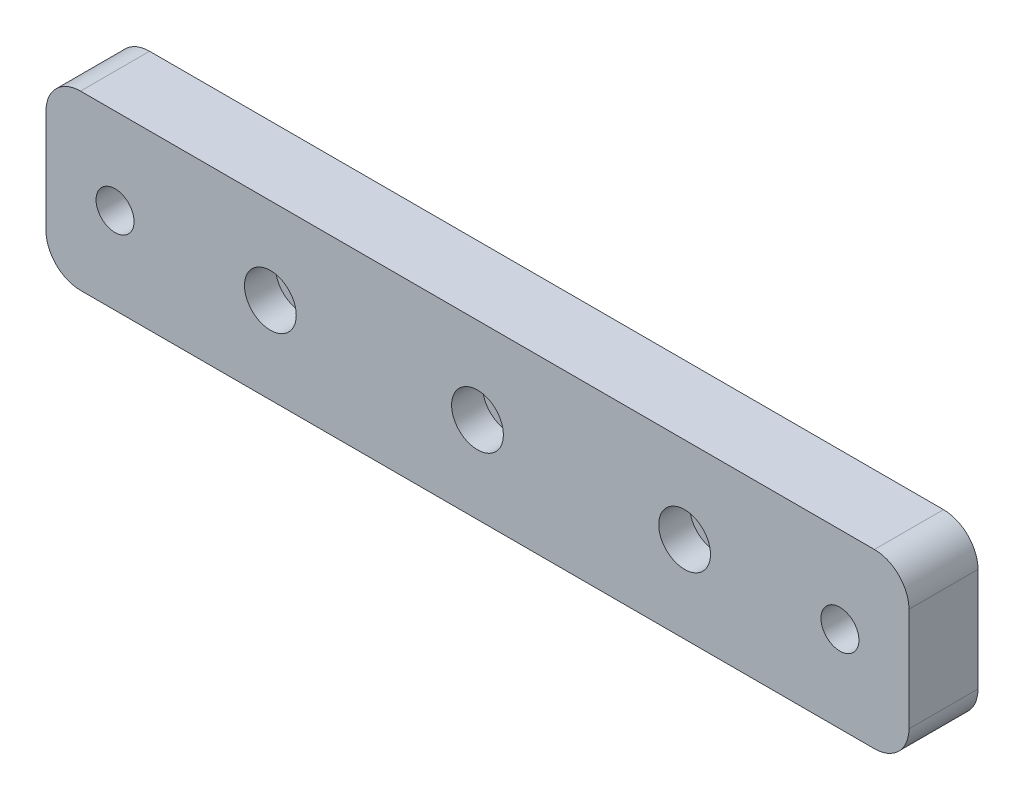
from build123d import *

# Parameters (mm, degrees)
SKETCH1_W                                    = 250
SKETCH1_H                                    = 50
BOSS_EXTRUDE1_DEPTH                          = 20
FILLET1_R                                    = 10
LPATTERN1_COUNT                              = 3
LPATTERN1_PITCH                              = 60
CBORE_FOR_M10_HEXAGON_SOCKET_HEAD_CA_2_COUNT = 2
CBORE_FOR_M10_HEXAGON_SOCKET_HEAD_CA_2_PITCH = 210


with BuildPart() as part:
    # Sketch1 → Boss-Extrude1 (new body)
    with BuildSketch(Plane.XY):
        with Locations((-50, 0)):
            Rectangle(SKETCH1_W, SKETCH1_H)
    extrude(amount=BOSS_EXTRUDE1_DEPTH)

    # Fillet1
    fillet1_edges = [part.edges().sort_by_distance(p)[0] for p in [
        (-175, 25, 10),
        (75, 25, 10),
        (75, -25, 10),
        (-175, -25, 10),
    ]]
    fillet(fillet1_edges, radius=FILLET1_R)

    # Sketch2 → CBORE for M8 Hexagon socket head cap screws1 (revolve, cut)
    with BuildSketch(Plane(origin=(10, 0, 20), x_dir=(0, -1, 0), z_dir=(1, 0, 0))):
        Polygon((0, 0), (0, 24.953872786), (4.5, 22.25), (4.5, 9), (7.5, 9), (7.5, 0), align=None)
    cbore_for_m8_hexagon_socket_head_cap_scr = revolve(axis=Axis((10, 0, 26.35), (0, 0, -1)), mode=Mode.SUBTRACT)

    # LPattern1: CBORE for M8 Hexagon socket head cap screws1 ×3
    with Locations(*[(-i * LPATTERN1_PITCH, 0, 0) for i in range(1, LPATTERN1_COUNT)]):
        add(cbore_for_m8_hexagon_socket_head_cap_scr, mode=Mode.SUBTRACT)

    # Sketch4 → CBORE for M10 Hexagon socket head cap screws1 (revolve, cut)
    with BuildSketch(Plane.YZ.offset(55)):
        Polygon((0, 0), (0, 30.804733405), (5.5, 27.5), (5.5, 11), (9, 11), (9, 0.025), (9.025, 0), align=None)
    cbore_for_m10_hexagon_socket_head_cap_sc = revolve(axis=Axis((55, 0, -6.35), (0, 0, 1)), mode=Mode.SUBTRACT)

    # CBORE for M10 Hexagon socket head ca 2: CBORE for M10 Hexagon socket head cap screws1 ×2
    with Locations(*[(-i * CBORE_FOR_M10_HEXAGON_SOCKET_HEAD_CA_2_PITCH, 0, 0) for i in range(1, CBORE_FOR_M10_HEXAGON_SOCKET_HEAD_CA_2_COUNT)]):
        add(cbore_for_m10_hexagon_socket_head_cap_sc, mode=Mode.SUBTRACT)


solid = part.part
